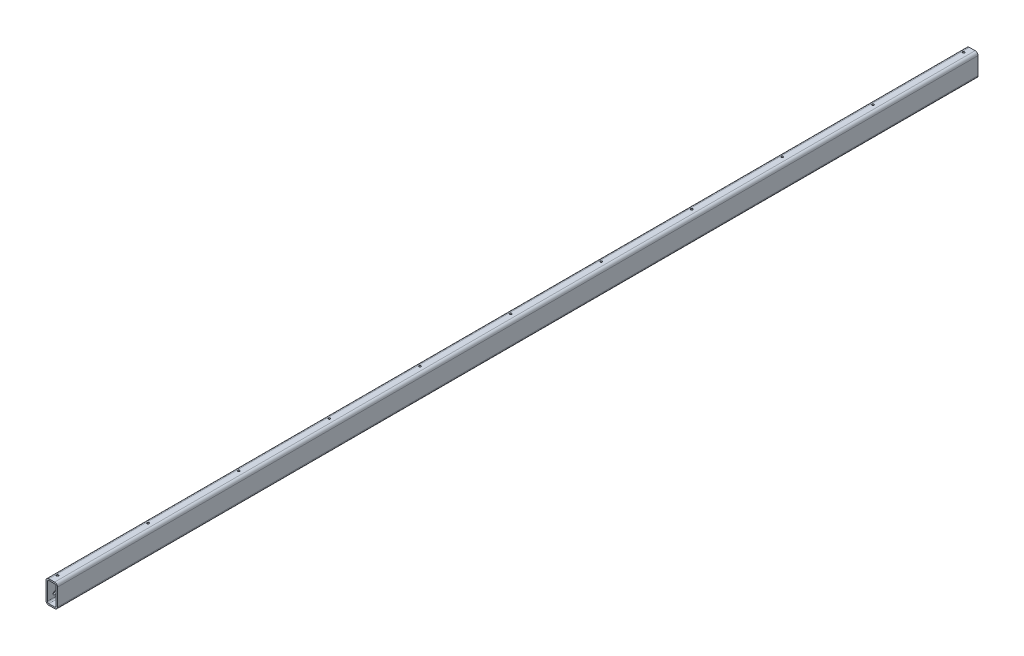
from build123d import *

# Parameters (mm, degrees)
BOSS_EXTRUDE1_DEPTH   = 3200
SKETCH_1_R            = 3.25
CUT_EXTRUDE1_DEPTH    = 10
M8_TAPPED_HOLE1_D     = 6.8
M8_TAPPED_HOLE1_DEPTH = 22.25
M8_TAPPED_HOLE1_TIP   = 2.042926105
SKETCH9_R             = 5.5
CUT_EXTRUDE2_DEPTH    = 10
LPATTERN1_COUNT       = 11
LPATTERN1_PITCH       = 315


with BuildPart() as part:
    # Sketch1 → Boss-Extrude1 (new body)
    with BuildSketch(Plane.XY):
        with BuildLine():
            Line((-10, -40), (10, -40))
            ThreePointArc((10, -40), (17.071067812, -37.071067812), (20, -30))
            Line((20, -30), (20, 30))
            ThreePointArc((20, 30), (17.071067812, 37.071067812), (10, 40))
            Line((10, 40), (-10, 40))
            ThreePointArc((-10, 40), (-17.071067812, 37.071067812), (-20, 30))
            Line((-20, 30), (-20, -30))
            ThreePointArc((-20, -30), (-17.071067812, -37.071067812), (-10, -40))
        make_face()
        with BuildLine():
            Line((-10, -35), (10, -35))
            ThreePointArc((10, -35), (13.535533906, -33.535533906), (15, -30))
            Line((15, -30), (15, 30))
            ThreePointArc((15, 30), (13.535533906, 33.535533906), (10, 35))
            Line((10, 35), (-10, 35))
            ThreePointArc((-10, 35), (-13.535533906, 33.535533906), (-15, 30))
            Line((-15, 30), (-15, -30))
            ThreePointArc((-15, -30), (-13.535533906, -33.535533906), (-10, -35))
        make_face(mode=Mode.SUBTRACT)
    extrude(amount=BOSS_EXTRUDE1_DEPTH)

    # 草图1 → Cut-Extrude1 (cut)
    with BuildSketch(Plane(origin=(0, 40, 0), x_dir=(1, 0, 0), z_dir=(0, 1, 0))):
        with Locations(Location((-5, -3175, 0), (0, 0, 270))):
            Circle(SKETCH_1_R)
        with Locations(Location((-5, -2860, 0), (0, 0, 270))):
            Circle(SKETCH_1_R)
        with Locations(Location((-5, -2545, 0), (0, 0, 270))):
            Circle(SKETCH_1_R)
        with Locations(Location((-5, -2230, 0), (0, 0, 270))):
            Circle(SKETCH_1_R)
        with Locations(Location((-5, -1915, 0), (0, 0, 270))):
            Circle(SKETCH_1_R)
        with Locations(Location((-5, -1600, 0), (0, 0, 270))):
            Circle(SKETCH_1_R)
        with Locations(Location((-5, -1285, 0), (0, 0, 270))):
            Circle(SKETCH_1_R)
        with Locations(Location((-5, -970, 0), (0, 0, 270))):
            Circle(SKETCH_1_R)
        with Locations(Location((-5, -655, 0), (0, 0, 270))):
            Circle(SKETCH_1_R)
        with Locations(Location((-5, -340, 0), (0, 0, 270))):
            Circle(SKETCH_1_R)
        with Locations(Location((-5, -25, 0), (0, 0, 270))):
            Circle(SKETCH_1_R)
    extrude(amount=-CUT_EXTRUDE1_DEPTH, mode=Mode.SUBTRACT)

    # M8 Tapped Hole1
    with Locations(Plane(origin=(0, 40, 0), x_dir=(1, 0, 0), z_dir=(0, 1, 0))):
        with Locations((-5, -3175), (-5, -2860), (-5, -2545), (-5, -2230), (-5, -1915), (-5, -1600), (-5, -1285), (-5, -970), (-5, -655), (-5, -340), (-5, -25)):
            Hole(M8_TAPPED_HOLE1_D / 2, depth=M8_TAPPED_HOLE1_DEPTH)
            with Locations((0, 0, -(M8_TAPPED_HOLE1_DEPTH + M8_TAPPED_HOLE1_TIP / 2))):  # 118° drill point
                Cone(0, M8_TAPPED_HOLE1_D / 2, M8_TAPPED_HOLE1_TIP, mode=Mode.SUBTRACT)

    # Sketch9 → Cut-Extrude2 (cut)
    with BuildSketch(Plane.ZY.offset(20)):
        with Locations((25, -17.5)):
            Circle(SKETCH9_R)
    cut_extrude2 = extrude(amount=-CUT_EXTRUDE2_DEPTH, mode=Mode.SUBTRACT)

    # LPattern1: Cut-Extrude2 ×11
    with Locations(*[(0, 0, i * LPATTERN1_PITCH) for i in range(1, LPATTERN1_COUNT)]):
        add(cut_extrude2, mode=Mode.SUBTRACT)


solid = part.part
